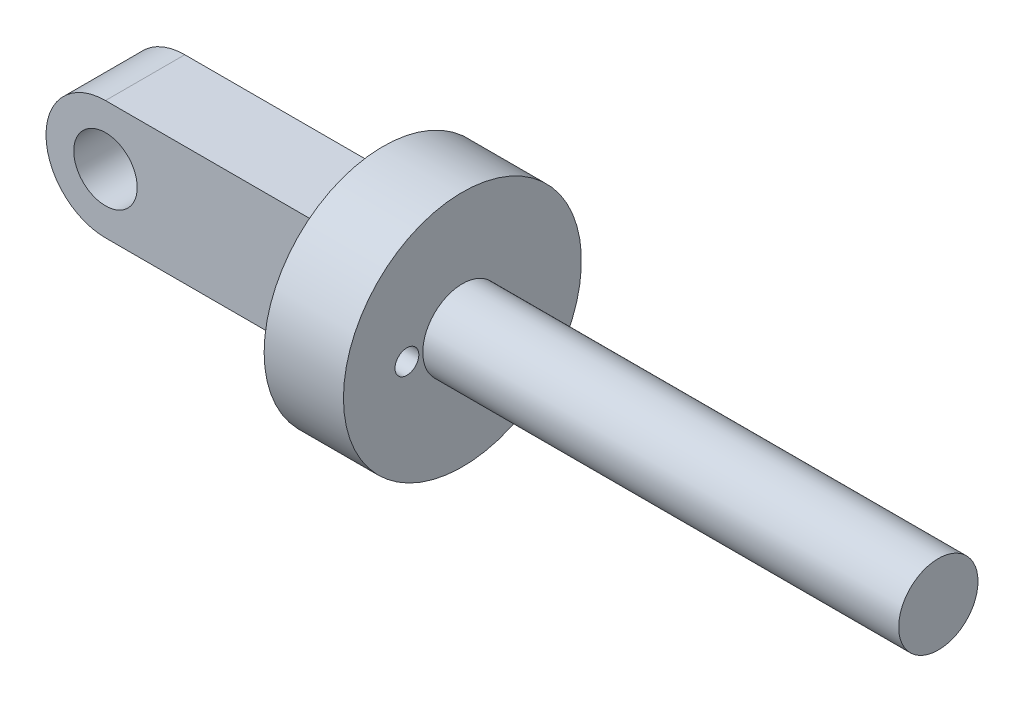
from build123d import *

# Parameters (mm, degrees)
SKETCH2_R           = 0.4
BOSS_EXTRUDE1_DEPTH = 0.5
SKETCH4_R           = 1
SKETCH4_R_2         = 0.5
CUT_EXTRUDE3_DEPTH  = 6
SKETCH5_R           = 0.15
CUT_EXTRUDE4_DEPTH  = 10


with BuildPart() as part:
    # Sketch1 → Revolve1 (revolve)
    with BuildSketch(Plane.XY, mode=Mode.PRIVATE) as revolve1_sk:
        Polygon((0, 0), (0, 1.5), (1, 1.5), (1, 1), (7, 1), (7, 0), align=None)
    revolve(revolve1_sk.sketch.rotate(Axis((0.124352332, 0, 0), (1, 0, 0)), 90), axis=Axis((0.124352332, 0, 0), (1, 0, 0)))

    # Sketch2 → Boss-Extrude1 (add, symmetric)
    with BuildSketch(Plane.XY):
        with BuildLine():
            Line((0, 0.75), (0, -0.75))
            Line((0, -0.75), (-3, -0.75))
            ThreePointArc((-3, -0.75), (-3.75, 0), (-3, 0.75))
            Line((-3, 0.75), (0, 0.75))
        make_face()
        with Locations((-3, 0)):
            Circle(SKETCH2_R, mode=Mode.SUBTRACT)
    extrude(amount=BOSS_EXTRUDE1_DEPTH, both=True)

    # Sketch4 → Cut-Extrude3 (cut)
    with BuildSketch(Plane(origin=(7, 0, 0), x_dir=(0, 0, -1), z_dir=(1, 0, 0))):
        Circle(SKETCH4_R)
        Circle(SKETCH4_R_2, mode=Mode.SUBTRACT)
    extrude(amount=-CUT_EXTRUDE3_DEPTH, mode=Mode.SUBTRACT)

    # Sketch5 → Cut-Extrude4 (cut)
    with BuildSketch(Plane.ZY):
        with Locations((0.7, 0)):
            Circle(SKETCH5_R)
    extrude(amount=-CUT_EXTRUDE4_DEPTH, mode=Mode.SUBTRACT)


solid = part.part
